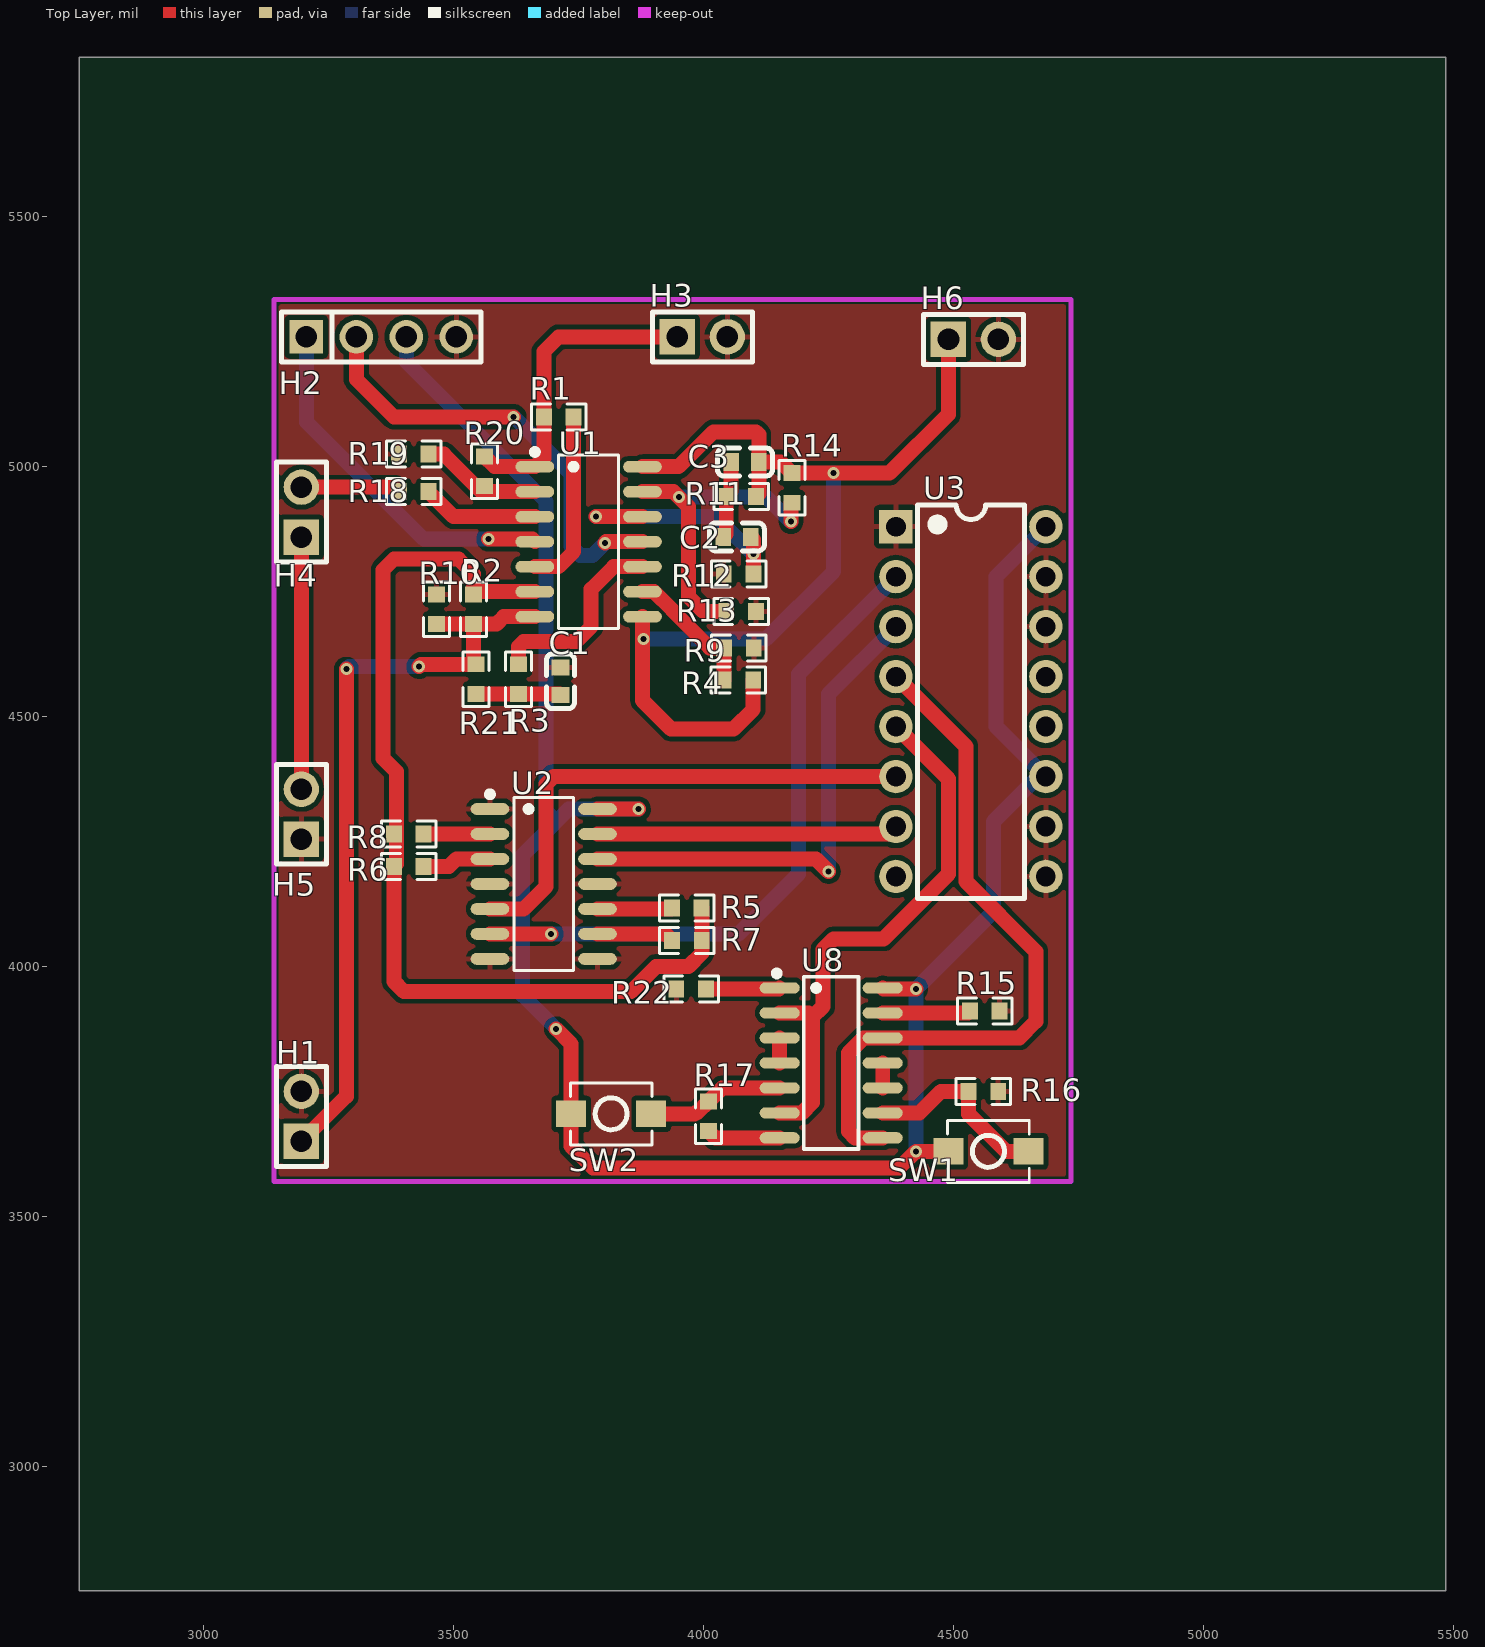
[diagram p0: Top Layer view]
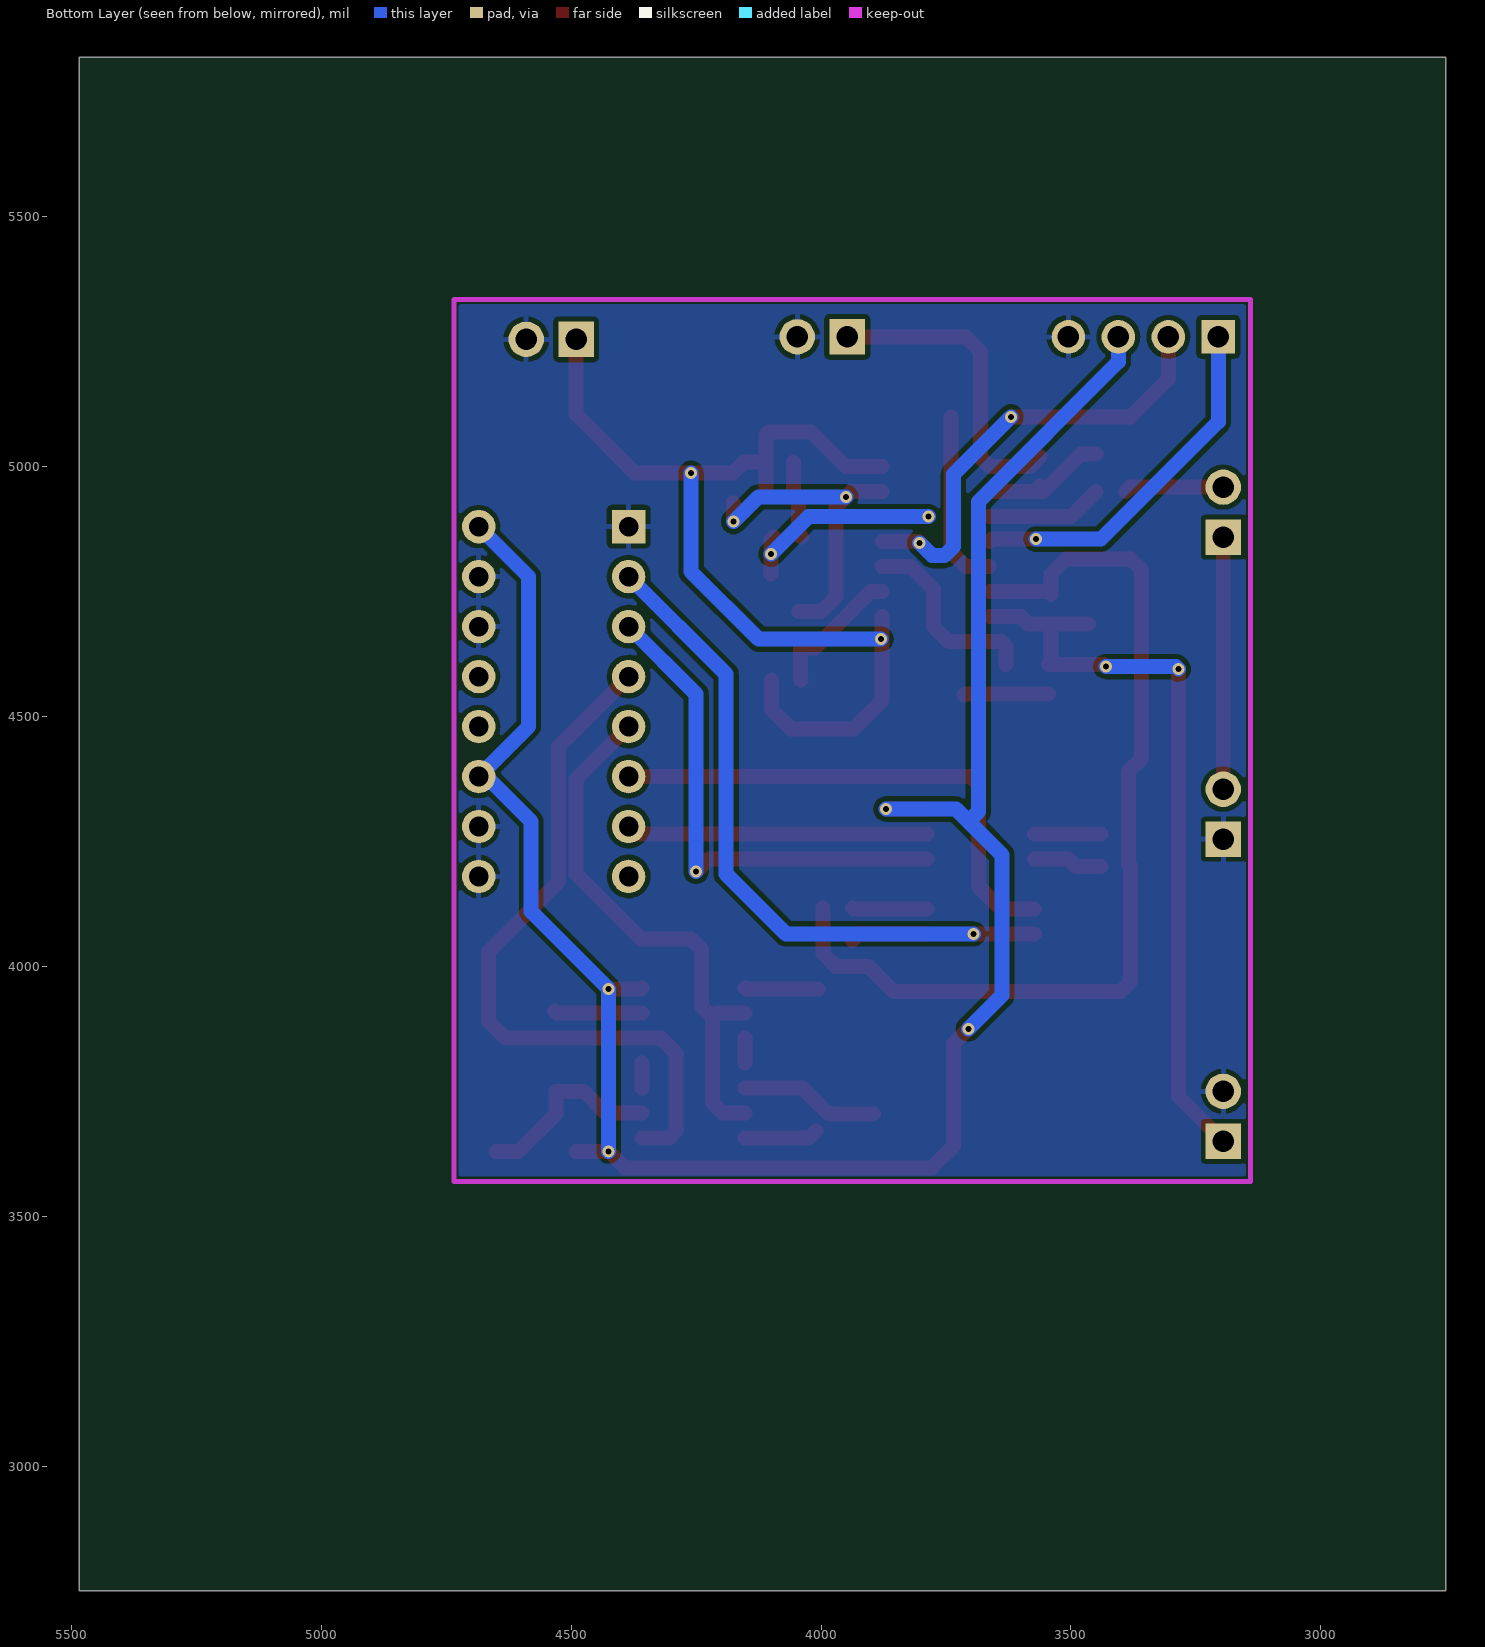
[diagram p1: Bottom Layer view, seen from below]
# Altium PCB MISC52000.pcbdoc
Units mil, origin at the board's own origin, x right, y up, seen from the top; angles counter-clockwise.
Board outline 2735 x 3070 mil, 2 copper layers (Top Layer, Bottom Layer), stack 62.206 mil thick; 37 components, 36 nets, 126 pads, 17 vias.

## Layer stack, top to bottom
Top Solder Mask Layer: solder mask 0.394, Dk 3.3
Top Layer: signal copper 1.379
Dielectric1: surface 59.449, FR4, Dk 4.5
Bottom Layer: signal copper 1.378
Bottom Solder Mask Layer: solder mask 0.394, Dk 3.3

## Board outline
5485,2750 2750,2750 2750,5820 5485,5820

## Design rules (kind name [scope] priority, off if disabled: settings)
BoardOutlineClearance copperThickness2oz_1 [All] p2 off: genericclearance=7.99 ignorepadtopadclearanceinfootprint=FALSE except(0: Arc-SplitContinuation Track-SplitContinuation SMDPad-SplitContinuation THPad-SplitContinuation Via-SplitContinuation Fill-SplitContinuation Region-SplitContinuation Poly-SplitContinuation Text-SplitContinuation Hole-SplitContinuation; 5.98: Arc-CutoutEdge SMDPad-CutoutEdge THPad-CutoutEdge Via-CutoutEdge Fill-CutoutEdge Region-CutoutEdge Text-CutoutEdge; 6.93: Hole-OutlineEdge Hole-CutoutEdge; 10: Poly-OutlineEdge Poly-CutoutEdge; 11.81: Arc-OutlineEdge Track-OutlineEdge SMDPad-OutlineEdge THPad-OutlineEdge Via-OutlineEdge Fill-OutlineEdge Region-OutlineEdge Text-OutlineEdge Track-CutoutEdge)
BoardOutlineClearance copperThickness1oz_1 [All] p4: genericclearance=4.02 ignorepadtopadclearanceinfootprint=FALSE except(0: Arc-SplitContinuation Track-SplitContinuation SMDPad-SplitContinuation THPad-SplitContinuation Via-SplitContinuation Fill-SplitContinuation Region-SplitContinuation Poly-SplitContinuation Text-SplitContinuation Hole-SplitContinuation; 6: SMDPad-CutoutEdge THPad-CutoutEdge Via-CutoutEdge Fill-CutoutEdge Region-CutoutEdge Text-CutoutEdge; 6.93: Hole-OutlineEdge Hole-CutoutEdge; 10: Poly-OutlineEdge Poly-CutoutEdge; 11.8: Arc-OutlineEdge Track-OutlineEdge SMDPad-OutlineEdge THPad-OutlineEdge Via-OutlineEdge Fill-OutlineEdge Region-OutlineEdge Text-OutlineEdge; 11.81: Arc-CutoutEdge Track-CutoutEdge)
Clearance copperThickness2oz [All] p1 off: gap=7.99 ignorepadtopadclearanceinfootprint=FALSE except(5.98: SMDPad-Track SMDPad-SMDPad THPad-Track SMDPad-THPad THPad-THPad Track-Via SMDPad-Via THPad-Via Via-Via Fill-Track Region-Track Fill-SMDPad Region-SMDPad Fill-THPad Region-THPad Fill-Via Region-Via Fill-Fill Fill-Region Region-Region Arc-Track Arc-SMDPad Arc-THPad Arc-Via Fill-Arc Region-Arc Arc-Arc Text-Track SMDPad-Text Text-THPad Text-Via Fill-Text Region-Text Arc-Text Text-Text; 6.93: Hole-Track Hole-SMDPad Hole-THPad Hole-Via Fill-Hole Region-Hole Hole-Arc Hole-Text; 10: Poly-Track Poly-SMDPad Poly-THPad Poly-Via Poly-Fill Poly-Region Poly-Poly Poly-Arc Poly-Text Poly-Hole)
Clearance copperThickness1oz [All] p3: gap=4.02 ignorepadtopadclearanceinfootprint=FALSE except(5.98: SMDPad-Track SMDPad-SMDPad THPad-Track SMDPad-THPad THPad-THPad Track-Via SMDPad-Via THPad-Via Via-Via Fill-Track Region-Track Fill-SMDPad Region-SMDPad Fill-THPad Region-THPad Fill-Via Region-Via Fill-Fill Fill-Region Region-Region; 6: Arc-Track Arc-SMDPad Arc-THPad Arc-Via Fill-Arc Region-Arc Arc-Arc Text-Track SMDPad-Text Text-THPad Text-Via Fill-Text Region-Text Arc-Text Text-Text; 6.93: Hole-Track Hole-SMDPad Hole-THPad Hole-Via Fill-Hole Region-Hole Hole-Arc Hole-Text; 10: Poly-Track Poly-SMDPad Poly-THPad Poly-Via Poly-Fill Poly-Region Poly-Poly Poly-Arc Poly-Text Poly-Hole)
DiffPairsRouting differentialPair [All] p1: maxlimit=6 minlimit=6 mostfreqgap=6 toplayer_minwidth=5 toplayer_prefwidth=10 toplayer_maxwidth=100 toplayer_mingap=6 toplayer_prefgap=6 toplayer_maxgap=6 bottomlayer_minwidth=5 bottomlayer_prefwidth=10 bottomlayer_maxwidth=100 bottomlayer_mingap=6 bottomlayer_prefgap=6 bottomlayer_maxgap=6 maxuncoupledlength=10
HoleToHoleClearance otherClearance [All] p1: gap=11.81 allowstackedmicrovias=TRUE
Length netLength [All] p1: minlimit=0 maxlimit=0
MatchedLengths netLengthTolerance [All] p1: tolerance=1000
PasteMaskExpansion pasteMaskExpansion [All] p1: expansion=0
PlaneConnect innerPlane [All] p1: planeconnectstyle=Relief reliefexpansion=20 reliefentries=4 reliefconductorwidth=10 reliefairgap=10
PolygonConnect copperRegion [(InNet('GND'))] p1: connectstyle=Relief reliefconductorwidth=10 reliefentries=4 polygonreliefangle="90 Angle" airgapwidth=10 via.connectstyle=Relief via.reliefconductorwidth=10 via.reliefentries=4 via.polygonreliefangle="90 Angle" via.airgapwidth=10
RoutingVias viaSize [All] p1: holewidth=12.01 width=24.02 viastyle="Through Hole" minholewidth=11.81 minwidth=19.68 maxholewidth=248.03 maxwidth=393.7
SolderMaskExpansion solderMaskExpansion [IsVia] p1: expansion=-1000 istentingtop=TRUE
SolderMaskExpansion solderMaskExpansion [All] p2: expansion=2 istentingtop=FALSE
Width copperThickness2oz_2 [All] p1 off: maxlimit=100 minlimit=8 preferedwidth=10
Width copperThickness1oz_2 [All] p2: maxlimit=100 minlimit=5 preferedwidth=10

## Components (designator, comment, footprint, x,y, rotation, side; value= is the part's Value field where it differs from the comment)
C1 "10nF" C0603 3713.52,4570.68 r270 top
C2 "100nF" C0603 4066.84,4859.56 r180 top
C3 "100nF" C0603 4082.84,5009.56 r0 top
H1 "" HDR-TH_2P-P2.54-V-M-1 3195,3700 r90 top
H2 "" HDR-TH_4P-P2.54-V-M 3355,5260 r0 top
H3 "" HDR-TH_2P-P2.54-V-M-1 3997.5,5260 r0 top
H4 "" HDR-TH_2P-P2.54-V-M-1 3195,4909.14 r90 top
H5 "" HDR-TH_2P-P2.54-V-M-1 3195,4304.57 r90 top
H6 "" HDR-TH_2P-P2.54-V-M-1 4540,5255 r0 top
R1 "15K" R0603 3710,5100 r0 top
R2 "1200K" R0603 3540,4715 r270 top
R3 "47K" R0603 3630,4575 r90 top
R4 "120K" R0603 4069.7,4573.12 r0 top
R5 "80K" R0603 3966.39,4117.32 r0 top
R6 "40K" R0603 3410,4200 r180 top
R7 "20K" R0603 3966.73,4052.32 r0 top
R8 "10K" R0603 3410,4265 r180 top
R9 "230K" R0603 4070.78,4637.72 r180 top
R10 "80K" R0603 3465,4715 r270 top
R11 "15K" R0603 4075,4940 r0 top
R12 "15K" R0603 4070,4785 r0 top
R13 "80K" R0603 4075,4710 r180 top
R14 "51K" R0603 4176.54,4957.58 r270 top
R15 "15K" R0603 4562.58,3910.48 r0 top
R16 "15K" R0603 4560,3750 r180 top
R17 "1K" R0603 4010,3700 r90 top
R18 "10K" R0603 3420,4950 r0 top
R19 "10K" R0603 3420,5025 r0 top
R20 "90K" R0603 3561.55,4990.76 r90 top
R21 "120K" R0603 3545,4575 r270 top
R22 "15K" R0603 3975,3955 r180 top
SW1 "" Key_SMD_3x4x2 4570,3630 r180 top
SW2 "" Key_SMD_3x4x2 3815,3705 r180 top
U1 "LM324ADR" SOP-14_L8.6-W3.9-P1.27-LS6.0-BL 3770,4850 r270 top
U2 "CD4066BD" SOP-14_L8.6-W3.9-P1.27-LS6.0-BL 3680,4165 r270 top
U3 "NTE74193" PDIP-16_L19.7-W6.6-P2.54-LS7.6-BL 4535,4530 r270 top
U8 "SN74LS00DR" SOIC-14_L8.7-W3.9-P1.27-LS6.0-BL 4255.44,3806.82 r270 top

## Footprints (in the part's own frame and the unit in brackets; to place one, negate y for a bottom-side part, rotate by r counter-clockwise, add the part's x,y. Pads: shape width x height; smd on the part's side, far side on the other; paste and mask are expansions set on the pad)
C0603 [mm]
  rect 0.8x0.9 smd: 1(-0.7,0) 2(0.7,0)
  silkscreen extent -1.39,-0.71 1.39,0.71
HDR-TH_2P-P2.54-V-M-1 [mm]
  rect 1.8x1.8 hole 1.1: 1(-1.27,0)
  round 1.8 hole 1.1: 2(1.27,0)
  silkscreen extent -2.54,-1.27 2.54,1.27
HDR-TH_4P-P2.54-V-M [mm]
  rect 1.7x1.7 hole 1.1: 1(-3.81,0)
  round 1.7 hole 1.1: 2(-1.27,0) 3(1.27,0) 4(3.81,0)
  silkscreen extent -5.08,-1.27 5.08,1.27
Key_SMD_3x4x2 [mm]
  rect 1.53x1.36 smd paste+0 mask+0.051: 1(-2.035,0) 2(2.035,0)
  silkscreen extent -2.08,-1.58 2.08,1.58
PDIP-16_L19.7-W6.6-P2.54-LS7.6-BL [mm]
  rect 1.7x1.7 hole 1: 1(-8.89,-3.81)
  round 1.7 hole 1: 2(-6.35,-3.81) 3(-3.81,-3.81) 4(-1.27,-3.81) 5(1.27,-3.81) 6(3.81,-3.81) 7(6.35,-3.81) 8(8.89,-3.81) 9(8.89,3.81) 10(6.35,3.81) 11(3.81,3.81) 12(1.27,3.81) 13(-1.27,3.81) 14(-3.81,3.81) 15(-6.35,3.81) 16(-8.89,3.81)
  silkscreen extent -10,-2.7 10,2.73
R0603 [mil]
  rect 31.75x34.02 smd paste-3937.01 mask+2: 1(-29.66,0) 2(29.66,0)
  silkscreen extent -55,-26 55,26
SOIC-14_L8.7-W3.9-P1.27-LS6.0-BL [mil]
  oval 22.6x80.24 smd: 1(-150,-103.11) 2(-100,-103.11) 3(-50,-103.11) 4(0,-103.11) 5(50,-103.11) 6(100,-103.11) 7(150,-103.11) 8(150,103.11) 9(100,103.11) 10(50,103.11) 11(0,103.11) 12(-50,103.11) 13(-100,103.11) 14(-150,103.11)
  silkscreen extent -185,-115 172,55
SOP-14_L8.6-W3.9-P1.27-LS6.0-BL [mm]
  oval 0.595x1.968 smd: 1(-3.81,-2.734) 2(-2.54,-2.734) 3(-1.27,-2.734) 4(0,-2.734) 5(1.27,-2.734) 6(2.54,-2.734) 7(3.81,-2.734) 8(3.81,2.734) 9(2.54,2.734) 10(1.27,2.734) 11(0,2.734) 12(-1.27,2.734) 13(-2.54,2.734) 14(-3.81,2.734)
  silkscreen extent -4.71,-2.88 4.4,1.52

## Via types
v1: diameter 24.02, hole 12, Top Layer to Bottom Layer, 17 vias

## Nets (pads, with @x,y where several pads share a name; then routed paths per layer and width w, separated by ;. In a path a pad name is that pad's centre, name@x,y a point inside that pad or via, vN(x,y) a via of type N, cw(c..) or ccw(c..) an arc to the next point about the centre after c; other vN are vias at no path point)
5V: H2.3 SW1.2 SW2.2 U2.14 U3.11 U3.16 U8.14 | length 4373.1
  Top Layer w30: v1(3705,3875) 3734.88,3845.12 SW2.2 3734.88,3640.12 3778.2,3596.8 4391.8,3596.8 v1(4425,3630) SW1.2 ; U2.14 v1(3870,4315) ; U8.14 4360.36,3955 v1(4425,3955)
  Bottom Layer w30: H2.3 3405,5210 3685,4930 3685,4310 3705,4290 ; v1(3705,3875) 3637.91,3942.09 3637.91,4222.91 3705,4290 ; v1(3870,4315) 3730,4315 3705,4290 ; v1(4425,3630) v1(4425,3955) 4580,4110 4580,4290 4670,4380 U3.11 4585,4480 4585,4780 U3.16
12V: H2.1 U1.4 | length 726.8
  Top Layer w30: v1(3570,4855) 3657.37,4855 U1.4
  Bottom Layer w30: H2.1 3205,5090 3440,4855 v1(3570,4855)
$1N60: R18.2 U1.3 | length 233.4
  Top Layer w30: R18.2 3499.66,4900 U1.3
$1N64: H4.2 R18.1 | length 199.1
  Top Layer w30: H4.2 3381.2,4959.14 R18.1
$1N65: H4.1 H5.2 | length 504.6
  Top Layer w30: H5.2 H4.1
$1N69: H3.1 R1.1 R20.2 U1.1 | length 626.5
  Top Layer w30: R20.2 3581.97,5000 U1.1 3680.34,5017.97 R1.1 3680.34,5230.34 3710,5260 H3.1
$1N70: R19.2 R20.1 U1.2 | length 259.5
  Top Layer w30: R19.2 3480,5025 3555,4950 R20.1@3572.65,4950 ; R20.1 R20.1@3572.65,4950 ; U1.2 R20.1@3572.65,4950
$1N71: R1.2 U1.5 | length 360.2
  Top Layer w30: U1.5 3710,4800 3740,4830 3740,5099.66 R1.2
$1N74: R8.1 U2.2 | length 132.7
  Top Layer w30: R8.1 U2.2
$1N76: U3.5 U8.2 U8.6 | length 1109.8
  Top Layer w30: U8.6 4196.82,3706.82 4217.57,3727.57 4217.57,3898.79 ; U8.2 4209.54,3906.82 4217.57,3898.79 ; U3.5 4490,4375 4490,4185 4360,4055 4260,4055 4238.79,4033.79 4238.79,3920 4217.57,3898.79
$1N77: U3.4 U8.8 U8.12 | length 1438
  Top Layer w30: U8.8 4303.18,3656.82 4290,3670 4290,3826.82 4320,3856.82 U8.12 4631.82,3856.82 4665,3890 4665,4030 4525,4170 4525,4440 U3.4
$1N81: U2.13 U3.7 | length 603.6
  Top Layer w30: U2.13 4370,4265 U3.7
$1N82: U2.5 U3.6 | length 1042.5
  Top Layer w30: U2.5 3640,4115 3685,4160 3685,4365 3700,4380 U3.6
$1N83: U2.6 U3.2 | length 1343.1
  Top Layer w30: U2.6 v1(3695,4065)
  Bottom Layer w30: v1(3695,4065) 4070,4065 4190,4185 4190,4585 U3.2
$1N84: U2.12 U3.3 | length 1018.6
  Top Layer w30: U2.12 4225,4215 v1(4250,4190)
  Bottom Layer w30: v1(4250,4190) 4250,4545 U3.3
$1N86: R7.1 U2.9 | length 154.7
  Top Layer w30: U2.9 3924.39,4065 R7.1
$1N87: R6.1 U2.3 | length 138.9
  Top Layer w30: R6.1 3490,4200 3505,4215 U2.3
$1N88: R5.1 U2.10 | length 150.1
  Top Layer w30: U2.10 3934.42,4115 R5.1
$1N90: R2.1 R5.2 R6.2 R7.2 R8.2 U1.6 | length 1951.2
  Top Layer w30: U1.6 3545.34,4750 R2.1 3540,4785 3510,4815 3380,4815 3358.79,4793.79 3358.79,4416.21 3385,4390 3385,4204.66 R6.2 3380.34,3969.66 3400,3950 3855,3950 3905,4000 3970,4000 3996.39,4026.39 R7.2 3996.39,4116.98 R5.2
$1N92: R3.2 U1.10 | length 393.2
  Top Layer w30: R3.2 3630,4640 3640,4650 3745,4650 3775,4680 3775,4755 3820,4800 U1.10
$1N93: C1.2 R3.1 R21.2 | length 169.4
  Top Layer w30: R21.2 R3.1 3711.31,4545.34 C1.2
$1N94: R4.1 R9.2 U1.9 | length 275.6
  Top Layer w30: U1.9 3900.89,4750 3937.34,4713.54 3937.34,4712.66 4012.28,4637.72 R9.2 4041.12,4574.2 R4.1
$1N97: H1.1 R2.2 R10.2 R21.1 U1.7 | length 1532.5
  Top Layer w30: H1.1 3285,3740 v1(3285,4595) ; v1(3430,4600) 3434.66,4604.66 R21.1 3540,4609.66 R2.2 ; R10.2 R2.2 ; U1.7 3600,4700 3585.34,4685.34 R2.2
  Bottom Layer w30: v1(3285,4595) 3290,4600 v1(3430,4600)
$1N98: C2.1 R12.2 U1.12 | length 515.4
  Top Layer w30: v1(3785,4900) U1.12 ; C2.1 4099.66,4854.31 R12.2
  Bottom Layer w30: v1(3785,4900) 4025,4900 v1(4100,4825)
$1N99: C2.2 C3.1 R11.1 | length 156.6
  Top Layer w30: C2.2 4045.34,4865.62 R11.1 4055.28,4949.94 C3.1
$1N103: R13.2 R14.2 U1.13 | length 656.1
  Top Layer w30: U1.13 3940,4950 v1(3950.48,4939.52) 3970,4920 3970,4740 4000,4710 R13.2 ; v1(4175,4890) 4175,4926.37 R14.2
  Bottom Layer w30: v1(3950.48,4939.52) 4125.48,4939.52 v1(4175,4890)
$1N104: C3.2 H6.1 R4.2 R11.2 R14.1 U1.8 U1.14 | length 2099.9
  Top Layer w30: U1.8 3877.63,4532.37 3935,4475 4060,4475 4099.36,4514.36 R4.2 ; U1.14 3950,5000 4020,5070 4105,5070 4110.4,5064.6 C3.2 ; R11.2 4110.4,4945.74 C3.2 ; H6.1 4490,5105 4372.24,4987.24 v1(4260,4987.24) R14.1 4154.22,5009.56 C3.2
  Bottom Layer w30: v1(3880,4655) 4125,4655 4260,4790 v1(4260,4987.24)
$1N106: R15.1 U8.13 | length 175.9
  Top Layer w30: U8.13 4529.26,3906.82 R15.1
$1N109: U8.10 U8.11 | length 50
  Top Layer w30: U8.10 U8.11
$1N110: R16.2 SW1.1 U8.9 | length 385.7
  Top Layer w30: U8.9 4431.82,3706.82 4475,3750 R16.2 4530.34,3704.66 4605,3630 SW1.1
$1N113: U8.3 U8.4 | length 50
  Top Layer w30: U8.4 U8.3
$1N114: R17.2 SW2.1 U8.5 | length 278.7
  Top Layer w30: SW2.1 3982.1,3705 3984.3,3707.2 3987.54,3707.2 R17.2 4037.16,3756.82 U8.5
$1N116: R17.1 U8.7 | length 147.9
  Top Layer w30: R17.1 4023.52,3656.82 U8.7
$1N118: R22.1 U8.1 | length 148.4
  Top Layer w30: R22.1 4150.51,3955 U8.1
-12V: H2.2 U1.11 | length 900
  Top Layer w30: H2.2 3305,5175 3380,5100 v1(3620,5100) ; v1(3802.5,4847.5) 3805,4850 U1.11
  Bottom Layer w30: v1(3620,5100) 3735,4985 3735,4840 3752.57,4822.43 3777.43,4822.43 v1(3802.5,4847.5)
GND: C1.1 H1.2 H2.4 H3.2 H5.1 H6.2 R9.1 R10.1 R12.1 R13.1 R15.2 R16.1 R19.1 R22.2 U2.1 U2.4 U2.7 U2.8 U2.11 U3.1 U3.9 U3.10 U3.14 U3.15
pads on no net: U3.8 U3.12 U3.13

## Polygon pours and split planes (outlines as drawn)
GND on Top Layer (solid, remove dead copper, pour order 0): 3000,5570 3000,3000 5235,3000 5235,5570
GND on Bottom Layer (solid, remove dead copper, pour order 2): 3035,5485 3035,3410 5095,3410 5095,5485

## Keep-outs
Board Outline Layer:
  lines w10: 3140,3570 3140,5335 4735,5335 4735,3570 3140,3570